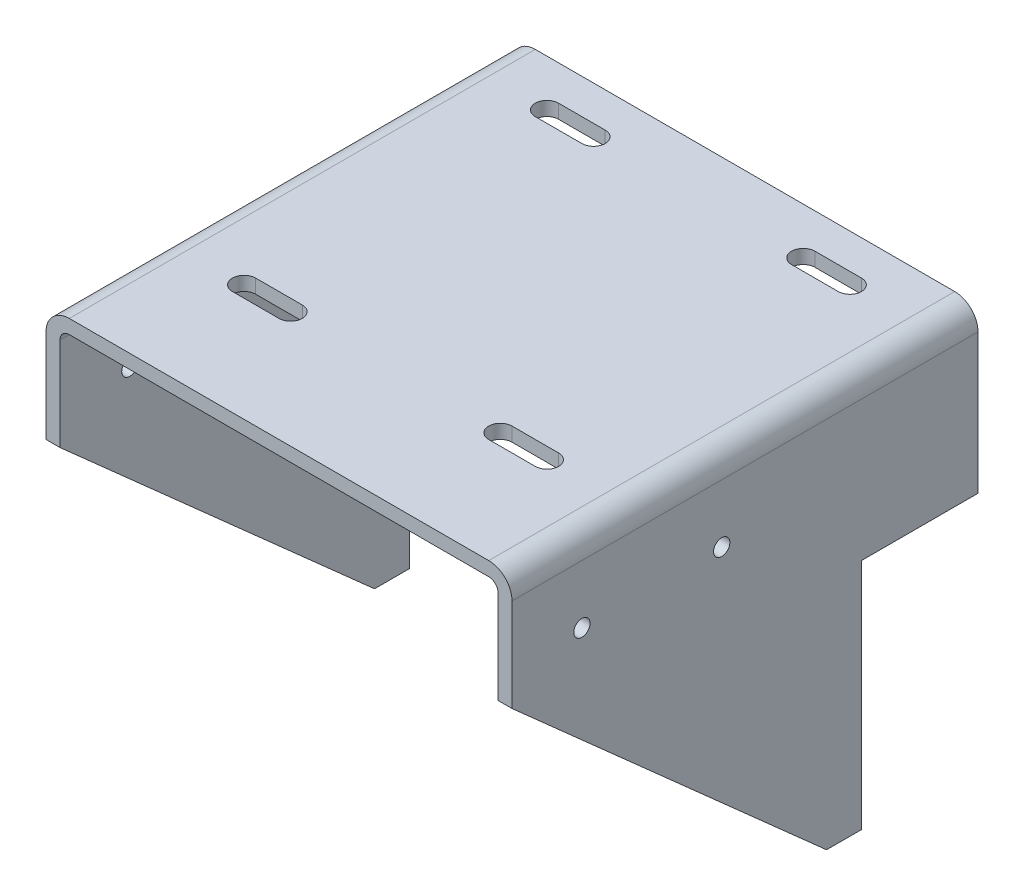
from build123d import *

# Parameters (mm, degrees)
BOSS_EXTRUDE2_DEPTH = 200
CUT_EXTRUDE1_DEPTH  = 200
SKETCH3_R           = 3.5
CUT_EXTRUDE2_DEPTH  = 200
CUT_EXTRUDE3_DEPTH  = 10


with BuildPart() as part:
    # Sketch1 → Boss-Extrude2 (new body)
    with BuildSketch(Plane.XY):
        with BuildLine():
            Line((0, 0), (0, 160))
            ThreePointArc((0, 160), (2.928932188, 167.071067812), (10, 170))
            Line((10, 170), (190, 170))
            ThreePointArc((190, 170), (197.071067812, 167.071067812), (200, 160))
            Line((200, 160), (200, 0))
            Line((200, 0), (194, 0))
            Line((194, 0), (194, 160))
            ThreePointArc((194, 160), (192.828427125, 162.828427125), (190, 164))
            Line((190, 164), (10, 164))
            ThreePointArc((10, 164), (7.171572875, 162.828427125), (6, 160))
            Line((6, 160), (6, 0))
            Line((6, 0), (0, 0))
        make_face()
    extrude(amount=BOSS_EXTRUDE2_DEPTH)

    # Sketch2 → Cut-Extrude1 (cut)
    with BuildSketch(Plane(origin=(200, 0, 0), x_dir=(0, 0, -1), z_dir=(1, 0, 0))):
        Polygon((-200, 120), (-65, 0), (-50, 0), (-50, 100), (0, 100), (0, -9.162692683), (-225.149686355, -7.960981017), (-227.038090402, 77.768418596), align=None)
    extrude(amount=-CUT_EXTRUDE1_DEPTH, mode=Mode.SUBTRACT)

    # Sketch3 → Cut-Extrude2 (cut)
    with BuildSketch(Plane(origin=(200, 0, 0), x_dir=(0, 0, -1), z_dir=(1, 0, 0))):
        with Locations(Location((-170, 135, 0), (0, 0, 90))):
            Circle(SKETCH3_R)
        with Locations(Location((-110, 135, 0), (0, 0, 90))):
            Circle(SKETCH3_R)
    extrude(amount=-CUT_EXTRUDE2_DEPTH, mode=Mode.SUBTRACT)

    # Sketch4 → Cut-Extrude3 (cut)
    with BuildSketch(Plane(origin=(0, 170, 0), x_dir=(1, 0, 0), z_dir=(0, 1, 0))):
        with BuildLine():
            Line((165, -25), (145, -25))
            ThreePointArc((145, -25), (140, -20), (145, -15))
            Line((145, -15), (165, -15))
            ThreePointArc((165, -15), (170, -20), (165, -25))
        make_face()
        with BuildLine():
            Line((165, -155), (145, -155))
            ThreePointArc((145, -155), (140, -150), (145, -145))
            Line((145, -145), (165, -145))
            ThreePointArc((165, -145), (170, -150), (165, -155))
        make_face()
        with BuildLine():
            Line((55, -25), (35, -25))
            ThreePointArc((35, -25), (30, -20), (35, -15))
            Line((35, -15), (55, -15))
            ThreePointArc((55, -15), (60, -20), (55, -25))
        make_face()
        with BuildLine():
            Line((55, -155), (35, -155))
            ThreePointArc((35, -155), (30, -150), (35, -145))
            Line((35, -145), (55, -145))
            ThreePointArc((55, -145), (60, -150), (55, -155))
        make_face()
    extrude(amount=-CUT_EXTRUDE3_DEPTH, mode=Mode.SUBTRACT)


solid = part.part
